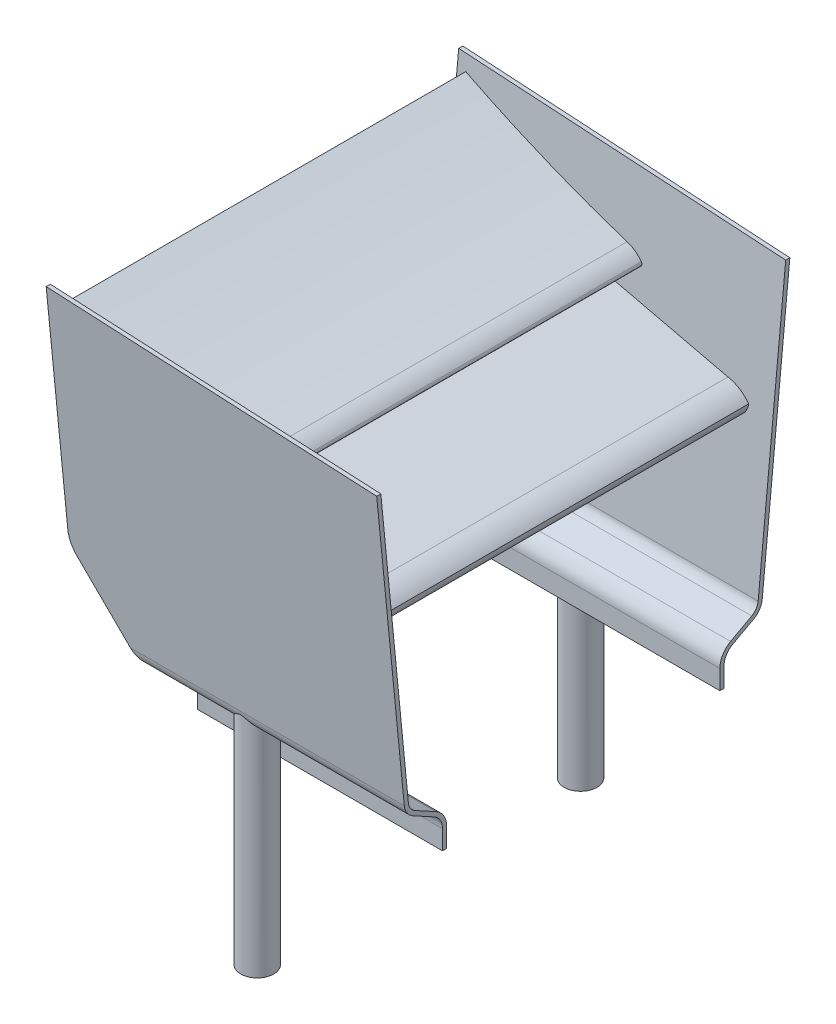
from build123d import *

# Parameters (mm, degrees)
SKETCH2_R                       = 2.54
BOSS_EXTRUDE1_DEPTH             = 38.1
BOSS_EXTRUDE2_DEPTH             = 25.4
BOSS_EXTRUDE2_DEPTH_BACK        = 25.4
CUT_EXTRUDE1_DEPTH              = 69.088
BOSS_EXTRUDE3_REACH             = 96.918
BOSS_EXTRUDE3_DIRECTION_2_REACH = 96.918
CUT_EXTRUDE2_DEPTH              = 95.917513418
CUT_EXTRUDE2_DEPTH_BACK         = 95.917513418


with BuildPart() as part:
    # Sketch2 → Boss-Extrude1 (new body)
    with BuildSketch(Plane(origin=(0, 0, 0), x_dir=(1, 0, 0), z_dir=(0, 1, 0))):
        with Locations(Location((0, -16.064088759, 0), (0, 0, 90))):
            Circle(SKETCH2_R)
    extrude(amount=BOSS_EXTRUDE1_DEPTH)

    # Sketch3 → Boss-Extrude2 (add, two sides: drawn at the far end of the back side and taken through both)
    with BuildSketch(Plane(origin=(0, 0, 0), x_dir=(0, 0, -1), z_dir=(1, 0, 0)).offset(-BOSS_EXTRUDE2_DEPTH_BACK)):
        with BuildLine():
            Line((-12.829078619, 26.300712117), (-12.829078619, 29.279919525))
            ThreePointArc((-12.829078619, 29.279919525), (-13.185613102, 30.577639963), (-14.155124552, 31.511043798))
            Line((-14.155124552, 31.511043798), (-17.42134678, 33.28819436))
            ThreePointArc((-17.42134678, 33.28819436), (-18.324951729, 34.116627002), (-18.735303364, 35.271795423))
            Line((-18.735303364, 35.271795423), (-23.274936915, 81.634267777))
            Line((-23.274936915, 81.634267777), (-22.642959252, 81.696148579))
            Line((-22.642959252, 81.696148579), (-18.103325701, 35.333676225))
            ThreePointArc((-18.103325701, 35.333676225), (-17.795561975, 34.467299909), (-17.117858263, 33.845975428))
            Line((-17.117858263, 33.845975428), (-13.851636036, 32.068824867))
            ThreePointArc((-13.851636036, 32.068824867), (-12.639746723, 30.902070072), (-12.194078619, 29.279919525))
            Line((-12.194078619, 29.279919525), (-12.194078619, 26.300712117))
            Line((-12.194078619, 26.300712117), (-12.829078619, 26.300712117))
        make_face()
    extrude(amount=BOSS_EXTRUDE2_DEPTH + BOSS_EXTRUDE2_DEPTH_BACK)

    # Sketch4 → Cut-Extrude1 (cut)
    with BuildSketch(Plane.ZY.offset(25.4)):
        with BuildLine():
            Line((18.518981342, 39.578693563), (18.103325701, 35.333676225))
            ThreePointArc((18.103325701, 35.333676225), (17.795561975, 34.467299909), (17.117858263, 33.845975428))
            Line((17.117858263, 33.845975428), (13.851636036, 32.068824867))
            ThreePointArc((13.851636036, 32.068824867), (12.639746723, 30.902070072), (12.194078619, 29.279919525))
            Line((12.194078619, 29.279919525), (9.661418427, 39.233443058))
            Line((9.661418427, 39.233443058), (18.518981342, 39.578693563))
        make_face()
    extrude(amount=-CUT_EXTRUDE1_DEPTH, mode=Mode.SUBTRACT)


with BuildPart() as body_2:
    # Mirror3: mirrored copy
    add(part.part.mirror(Plane.XY.offset(-8.916811241)))


with BuildPart() as part_1:
    add(part.part)

    add(body_2.part)  # Boss-Extrude3 merges body 2
    # Boss-Extrude3: up to this plane
    boss_extrude3_end = Plane(origin=(-25.4, 81.696148579, 22.642959252), z_dir=(0, -0.09745008287838285, 0.9952404138433066))
    # Sketch7 → Boss-Extrude3 (add, up to the surface)
    with BuildSketch(Plane.XY, mode=Mode.PRIVATE) as boss_extrude3_sk1:
        with BuildLine():
            Line((-7.043742341, 65.854012335), (18.267742921, 60.530914923))
            ThreePointArc((18.267742921, 60.530914923), (20.11486758, 59.911446579), (21.640598099, 58.699936398))
            ThreePointArc((21.640598099, 58.699936398), (21.489537489, 58.003085292), (21.14747004, 57.377457102))
            ThreePointArc((21.14747004, 57.377457102), (18.914053882, 56.866019856), (16.629775134, 57.044307226))
            ThreePointArc((16.629775134, 57.044307226), (4.513238392, 60.697337852), (-7.043742341, 65.854012335))
        make_face()
    boss_extrude3_tool1 = split(extrude(boss_extrude3_sk1.sketch, amount=BOSS_EXTRUDE3_REACH, mode=Mode.PRIVATE), bisect_by=boss_extrude3_end, keep=Keep.BOTH, mode=Mode.PRIVATE)
    add(boss_extrude3_tool1.solids().sort_by_distance((10.084711, 60.694895, 0))[0])
    # Sketch7 → Boss-Extrude3 (add, up to the surface)
    with BuildSketch(Plane.XY, mode=Mode.PRIVATE) as boss_extrude3_sk2:
        with BuildLine():
            ThreePointArc((-24.090462047, 79.298055074), (-11.317996693, 74.177627192), (1.76561715, 69.914564711))
            ThreePointArc((1.76561715, 69.914564711), (3.040960958, 69.370444609), (4.109363257, 68.486654453))
            ThreePointArc((4.109363257, 68.486654453), (4.217484646, 68.183885083), (4.079808176, 67.893360185))
            ThreePointArc((4.079808176, 67.893360185), (2.986644186, 67.343634533), (1.766311851, 67.433048138))
            ThreePointArc((1.766311851, 67.433048138), (-11.421869926, 72.799394657), (-24.090462047, 79.298055074))
        make_face()
    boss_extrude3_tool2 = split(extrude(boss_extrude3_sk2.sketch, amount=BOSS_EXTRUDE3_REACH, mode=Mode.PRIVATE), bisect_by=boss_extrude3_end, keep=Keep.BOTH, mode=Mode.PRIVATE)
    add(boss_extrude3_tool2.solids().sort_by_distance((-6.156417, 71.59743, 0))[0])

    # Boss-Extrude3 direction 2: up to this plane
    boss_extrude3_direction_2_end = Plane(origin=(-25.4, 81.696148579, -40.476581735), z_dir=(0, -0.09745008287838285, -0.9952404138433066))
    # Sketch7 → Boss-Extrude3 direction 2 (add, up to the surface)
    with BuildSketch(Plane.XY, mode=Mode.PRIVATE) as boss_extrude3_direction_2_sk1:
        with BuildLine():
            Line((-7.043742341, 65.854012335), (18.267742921, 60.530914923))
            ThreePointArc((18.267742921, 60.530914923), (20.11486758, 59.911446579), (21.640598099, 58.699936398))
            ThreePointArc((21.640598099, 58.699936398), (21.489537489, 58.003085292), (21.14747004, 57.377457102))
            ThreePointArc((21.14747004, 57.377457102), (18.914053882, 56.866019856), (16.629775134, 57.044307226))
            ThreePointArc((16.629775134, 57.044307226), (4.513238392, 60.697337852), (-7.043742341, 65.854012335))
        make_face()
    boss_extrude3_direction_2_tool1 = split(extrude(boss_extrude3_direction_2_sk1.sketch, amount=-BOSS_EXTRUDE3_DIRECTION_2_REACH, mode=Mode.PRIVATE), bisect_by=boss_extrude3_direction_2_end, keep=Keep.BOTH, mode=Mode.PRIVATE)
    add(boss_extrude3_direction_2_tool1.solids().sort_by_distance((10.084711, 60.694895, 0))[0])
    # Sketch7 → Boss-Extrude3 direction 2 (add, up to the surface)
    with BuildSketch(Plane.XY, mode=Mode.PRIVATE) as boss_extrude3_direction_2_sk2:
        with BuildLine():
            ThreePointArc((-24.090462047, 79.298055074), (-11.317996693, 74.177627192), (1.76561715, 69.914564711))
            ThreePointArc((1.76561715, 69.914564711), (3.040960958, 69.370444609), (4.109363257, 68.486654453))
            ThreePointArc((4.109363257, 68.486654453), (4.217484646, 68.183885083), (4.079808176, 67.893360185))
            ThreePointArc((4.079808176, 67.893360185), (2.986644186, 67.343634533), (1.766311851, 67.433048138))
            ThreePointArc((1.766311851, 67.433048138), (-11.421869926, 72.799394657), (-24.090462047, 79.298055074))
        make_face()
    boss_extrude3_direction_2_tool2 = split(extrude(boss_extrude3_direction_2_sk2.sketch, amount=-BOSS_EXTRUDE3_DIRECTION_2_REACH, mode=Mode.PRIVATE), bisect_by=boss_extrude3_direction_2_end, keep=Keep.BOTH, mode=Mode.PRIVATE)
    add(boss_extrude3_direction_2_tool2.solids().sort_by_distance((-6.156417, 71.59743, 0))[0])

    # Sketch8 → Cut-Extrude2 (cut, two sides: drawn at the far end of the back side and taken through both)
    with BuildSketch(Plane.XY.offset(-CUT_EXTRUDE2_DEPTH_BACK)):
        with BuildLine():
            Line((-24.256668996, 44.264399282), (-13.574711516, 31.167433557))
            ThreePointArc((-13.574711516, 31.167433557), (-12.725741657, 29.660795109), (-12.431380512, 27.956664612))
            Line((-12.431380512, 27.956664612), (-12.431380512, 22.730802701))
            Line((-12.431380512, 22.730802701), (-29.072503536, 23.334912896))
            Line((-29.072503536, 23.334912896), (-36.847334231, 46.202061997))
            Line((-36.847334231, 46.202061997), (-43.885114332, 82.767624865))
            Line((-43.885114332, 82.767624865), (28.390353763, 84.309501518))
            Line((28.390353763, 84.309501518), (29.354026671, 78.623831361))
            Line((29.354026671, 78.623831361), (-25.4, 81.634267777))
            Line((-25.4, 81.634267777), (-25.4, 51.141366203))
            Line((-25.4, 51.141366203), (-25.4, 47.475168227))
            ThreePointArc((-25.4, 47.475168227), (-25.105638855, 45.77103773), (-24.256668996, 44.264399282))
        make_face()
    extrude(amount=CUT_EXTRUDE2_DEPTH + CUT_EXTRUDE2_DEPTH_BACK, mode=Mode.SUBTRACT)


solid = part_1.part
